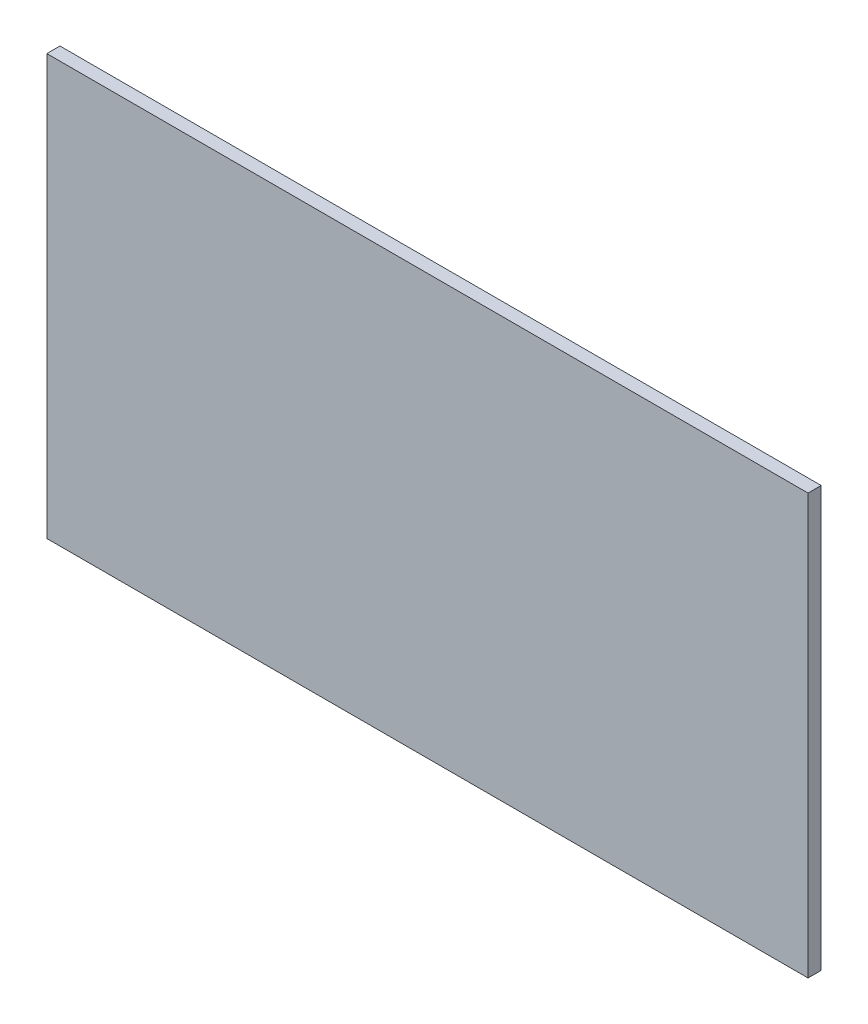
SolidWorks part; units mm, degrees
ref_plane "前视基准面" through (0, 0, 0) normal (0, 0, 1) x (1, 0, 0)
ref_plane "上视基准面" through (0, 0, 0) normal (0, 1, 0) x (1, 0, 0)
ref_plane "右视基准面" through (0, 0, 0) normal (1, 0, 0) x (0, 0, -1)
other "Configuration Table"
sketch "草图1" plane through (0, 0, 0) normal (0, 0, 1) x (1, 0, 0)
  line L0 (-29, -16) -> (29, -16)
  line L1 (29, -16) -> (29, 16)
  line L2 (29, 16) -> (-29, 16)
  line L3 (-29, 16) -> (-29, -16)
  point P0 (0, 0)
  dimension "D1" = 29
  dimension "D2" = 58
  dimension "D3" = 16
  dimension "D4" = 32
extrude "凸台-拉伸1" add sketch "草图1" against normal mid plane 1
